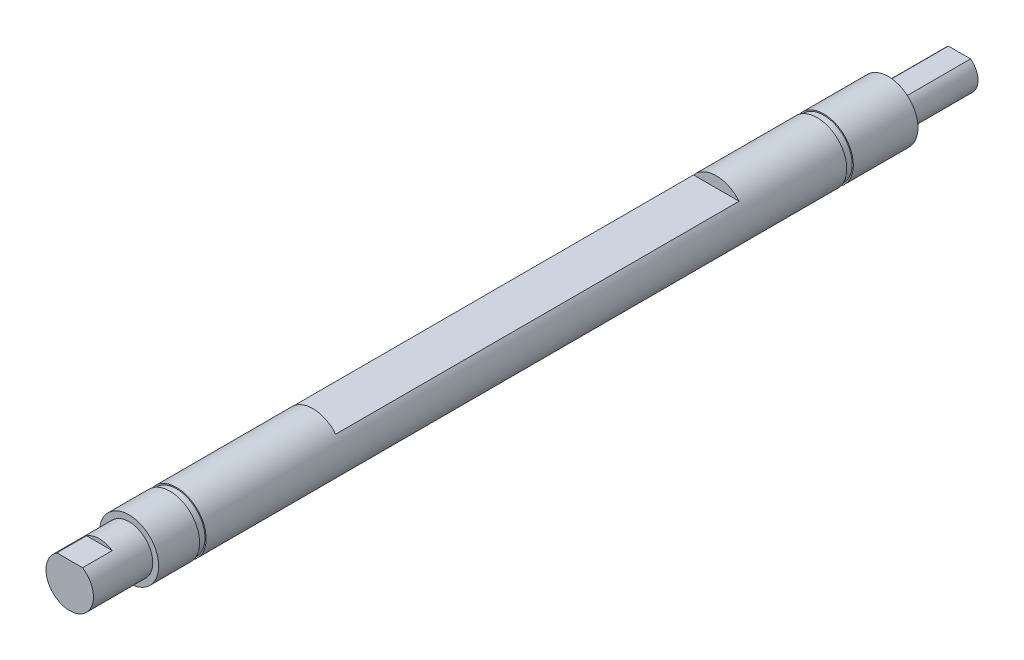
from build123d import *

# Parameters (mm, degrees)
SKETCH1_R               = 5
BOSS_EXTRUDE1_DEPTH     = 75
CUT_EXTRUDE1_DEPTH      = 76.332595867
CUT_EXTRUDE1_DEPTH_BACK = 76.332595867
SKETCH2_W               = 68
SKETCH2_H               = 14.535467824
CUT_EXTRUDE2_START      = -12
SKETCH3_R               = 5
SKETCH3_R_2             = 3.125
CUT_EXTRUDE2_DEPTH      = 12
SKETCH4_OUTSIDE_W       = 42.134
SKETCH4_OUTSIDE_H       = 42.134
CUT_EXTRUDE3_DEPTH      = 12
SKETCH5_OUTSIDE_W       = 42.134
SKETCH5_OUTSIDE_H       = 42.134
SKETCH5_OUTSIDE_R       = 4
CUT_EXTRUDE4_DEPTH      = 10
SKETCH6_W               = 10.564036003
SKETCH6_H               = 1.244008039
CUT_EXTRUDE5_DEPTH      = 5
SKETCH31_W              = 1.1
SKETCH31_H              = 0.2
SKETCH32_W              = 1.1
SKETCH32_H              = 0.2


with BuildPart() as part:
    # Sketch1 → Boss-Extrude1 (new, symmetric)
    with BuildSketch(Plane.XY):
        Circle(SKETCH1_R)
    extrude(amount=BOSS_EXTRUDE1_DEPTH, both=True)

    # Sketch2 → Cut-Extrude1 (cut, two sides: drawn at the far end of the back side and taken through both)
    with BuildSketch(Plane(origin=(0, 0, 0), x_dir=(0, 0, -1), z_dir=(1, 0, 0)).offset(-CUT_EXTRUDE1_DEPTH_BACK)):
        with Locations((0, 10.467733912)):
            Rectangle(SKETCH2_W, SKETCH2_H)
    extrude(amount=CUT_EXTRUDE1_DEPTH + CUT_EXTRUDE1_DEPTH_BACK, mode=Mode.SUBTRACT)

    # Sketch3 → Cut-Extrude2 (cut)
    with BuildSketch(Plane(origin=(0, 0, -75), x_dir=(-1, 0, 0), z_dir=(0, 0, -1)).offset(CUT_EXTRUDE2_START)):
        Circle(SKETCH3_R)
        Circle(SKETCH3_R_2, mode=Mode.SUBTRACT)
    extrude(amount=CUT_EXTRUDE2_DEPTH, mode=Mode.SUBTRACT)

    # Sketch4 outside → Cut-Extrude3 (cut)
    with BuildSketch(Plane(origin=(0, 0, -75), x_dir=(-1, 0, 0), z_dir=(0, 0, -1))):
        Rectangle(SKETCH4_OUTSIDE_W, SKETCH4_OUTSIDE_H)
        with BuildLine():
            Line((-1.957198253, 2.5), (1.957198253, 2.5))
            ThreePointArc((1.957198253, 2.5), (0, -3.175), (-1.957198253, 2.5))
        make_face(mode=Mode.SUBTRACT)
    extrude(amount=-CUT_EXTRUDE3_DEPTH, mode=Mode.SUBTRACT)

    # Sketch5 outside → Cut-Extrude4 (cut)
    with BuildSketch(Plane.XY.offset(75)):
        Rectangle(SKETCH5_OUTSIDE_W, SKETCH5_OUTSIDE_H)
        Circle(SKETCH5_OUTSIDE_R, mode=Mode.SUBTRACT)
    extrude(amount=-CUT_EXTRUDE4_DEPTH, mode=Mode.SUBTRACT)

    # Sketch6 → Cut-Extrude5 (cut)
    with BuildSketch(Plane.XY.offset(75)):
        with Locations((0.265856556, 3.982832188)):
            Rectangle(SKETCH6_W, SKETCH6_H)
    extrude(amount=-CUT_EXTRUDE5_DEPTH, mode=Mode.SUBTRACT)

    # Sketch31 → Cut-Revolve1 (revolve, cut)
    with BuildSketch(Plane(origin=(-100, 0, -63), x_dir=(0, 0, 1), z_dir=(0, 1, 0))):
        with Locations((11.45, 95.1)):
            Rectangle(SKETCH31_W, SKETCH31_H)
    revolve(axis=Axis((0, 0, -63), (0, 0, 1)), mode=Mode.SUBTRACT)

    # Sketch32 → Cut-Revolve11 (revolve, cut)
    with BuildSketch(Plane(origin=(100, 0, 65), x_dir=(0, 0, -1), z_dir=(0, 1, 0)), mode=Mode.PRIVATE) as cut_revolve11_sk:
        with Locations((7.45, 95.1)):
            Rectangle(SKETCH32_W, SKETCH32_H)
    revolve(cut_revolve11_sk.sketch.rotate(Axis((0, 0, 65), (0, 0, -1)), 180), axis=Axis((0, 0, 65), (0, 0, -1)), mode=Mode.SUBTRACT)


solid = part.part
